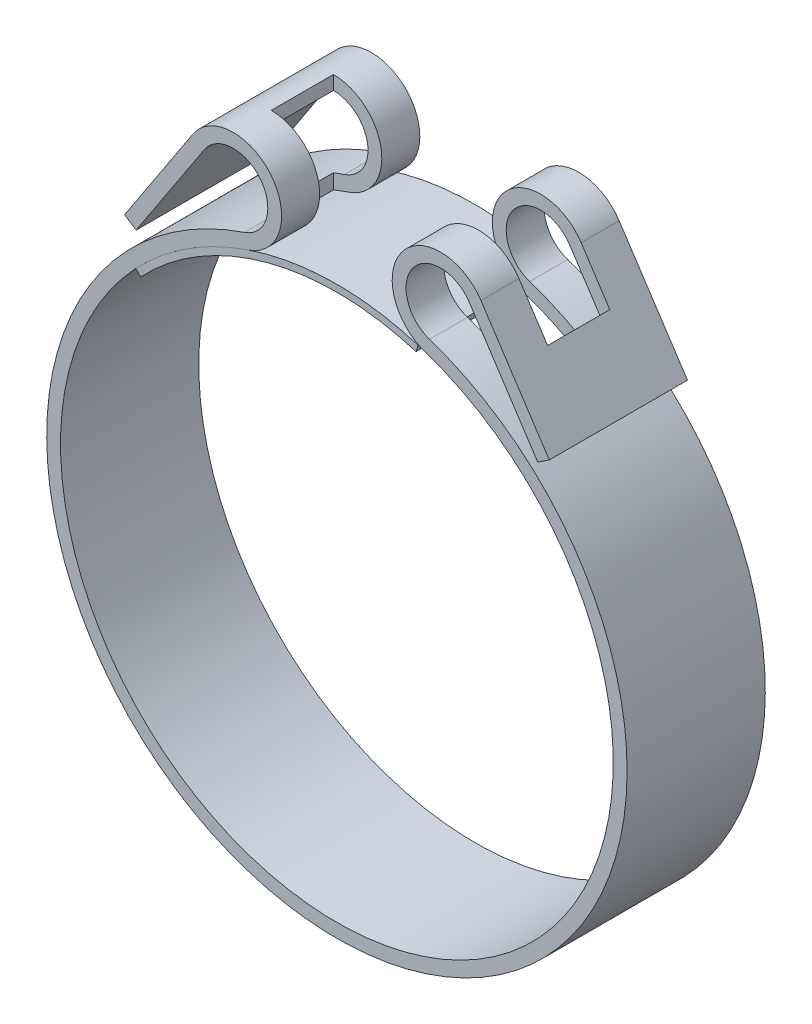
from build123d import *

# Parameters (mm, degrees)
EXTRUDE_1_DEPTH     = 20
SKETCH_3_W          = 20
SKETCH_3_H          = 9
CUT_EXTRUDE_1_DEPTH = 60
SKETCH_4_W          = 25
SKETCH_4_H          = 9
CUT_EXTRUDE_2_DEPTH = 60
EXTRUDE_2_DEPTH     = 20


with BuildPart() as part:
    # 草图1 → 凸台-拉伸1 (new body)
    with BuildSketch(Plane.XY):
        with BuildLine():
            Line((19.178255175, 47.288418545), (29.064948286, 32.246699915))
            Line((29.064948286, 32.246699915), (30.736250356, 33.345221372))
            Line((30.736250356, 33.345221372), (20.849557245, 48.386940001))
            ThreePointArc((20.849557245, 48.386940001), (9.45752093, 48.81773483), (12.765957447, 37.908182896))
            ThreePointArc((12.765957447, 37.908182896), (0, -40), (-12.765957447, 37.908182896))
            ThreePointArc((-12.765957447, 37.908182896), (-9.45752093, 48.81773483), (-20.849557245, 48.386940001))
            Line((-20.849557245, 48.386940001), (-30.736250356, 33.345221372))
            Line((-30.736250356, 33.345221372), (-29.064948286, 32.246699915))
            Line((-29.064948286, 32.246699915), (-19.178255175, 47.288418545))
            ThreePointArc((-19.178255175, 47.288418545), (-11.041086379, 47.596129136), (-13.404255319, 39.803592041))
            ThreePointArc((-13.404255319, 39.803592041), (0, -42), (13.404255319, 39.803592041))
            ThreePointArc((13.404255319, 39.803592041), (11.041086379, 47.596129136), (19.178255175, 47.288418545))
        make_face()
    extrude(amount=EXTRUDE_1_DEPTH)

    # 草图3 → 切除-拉伸1 (cut)
    with BuildSketch(Plane(origin=(0, 0, 0), x_dir=(1, 0, 0), z_dir=(0, 1, 0))):
        with Locations((-5, -10)):
            Rectangle(SKETCH_3_W, SKETCH_3_H)
    extrude(amount=CUT_EXTRUDE_1_DEPTH, mode=Mode.SUBTRACT)

    # 草图4 → 切除-拉伸2 (cut)
    with BuildSketch(Plane(origin=(0, 51.542114903, 0), x_dir=(1, 0, 0), z_dir=(0, 1, 0))):
        with Locations((12.5, -10)):
            Rectangle(SKETCH_4_W, SKETCH_4_H)
    extrude(amount=-CUT_EXTRUDE_2_DEPTH, mode=Mode.SUBTRACT)


with BuildPart() as body_2:
    # 草图5 → 凸台-拉伸2 (new body)
    with BuildSketch(Plane.XY):
        with BuildLine():
            Line((-28.389948704, 26.739686097), (-29.117896107, 27.425319074))
            ThreePointArc((-29.117896107, 27.425319074), (-10.228570764, 38.6700962), (11.750112977, 38.235256571))
            Line((11.750112977, 38.235256571), (11.456360153, 37.279375156))
            ThreePointArc((11.456360153, 37.279375156), (-9.972856495, 37.703343795), (-28.389948704, 26.739686097))
        make_face()
    extrude(amount=EXTRUDE_2_DEPTH)


solid = Compound([part.part, body_2.part])
